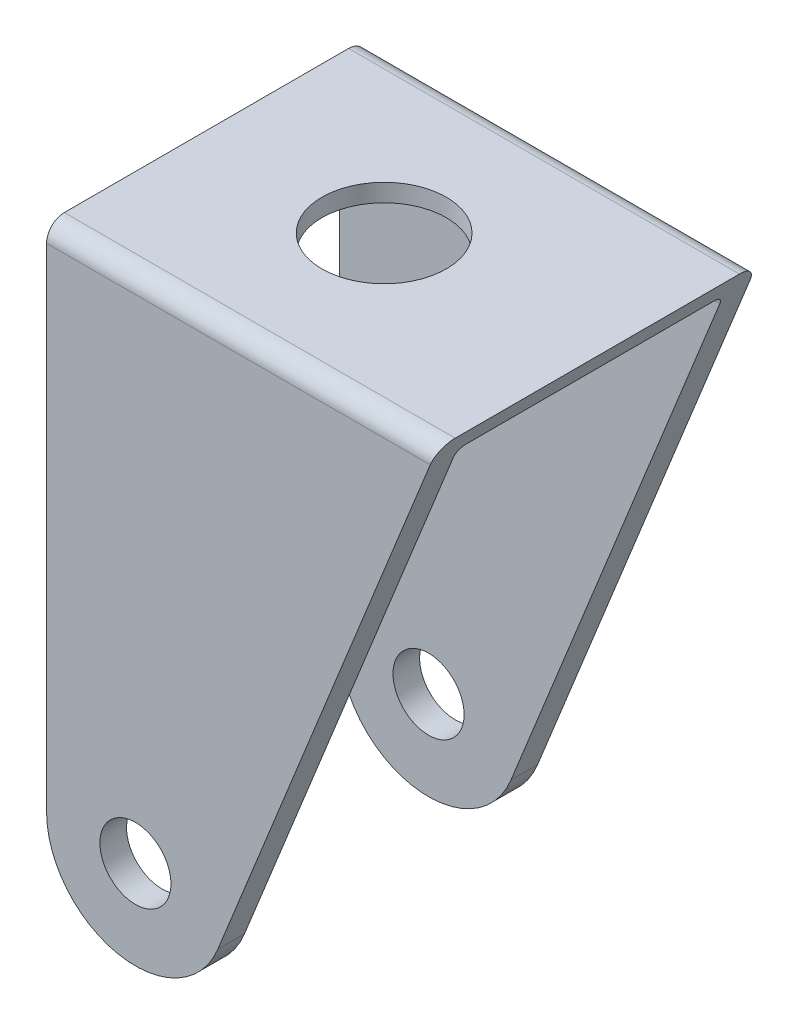
from build123d import *

# Parameters (mm, degrees)
SKETCH1_R           = 4
BOSS_EXTRUDE1_DEPTH = 36
CUT_EXTRUDE1_DEPTH  = 57
FILLET1_R           = 2
SKETCH3_R           = 7
CUT_EXTRUDE2_DEPTH  = 57


with BuildPart() as part:
    # Sketch1 → Boss-Extrude1 (new body)
    with BuildSketch(Plane.XY):
        with BuildLine():
            Line((0, 0), (0, -57.458281391))
            ThreePointArc((0, -57.458281391), (8.091910046, -67.274553225), (19.271838546, -61.204347325))
            Line((19.271838546, -61.204347325), (44, 0))
            Line((44, 0), (0, 0))
        make_face()
        with Locations((10, -57.458281391)):
            Circle(SKETCH1_R, mode=Mode.SUBTRACT)
    extrude(amount=-BOSS_EXTRUDE1_DEPTH)

    # Sketch2 → Cut-Extrude1 (cut)
    with BuildSketch(Plane.ZY):
        with BuildLine():
            Line((-32, -2), (-4, -2))
            ThreePointArc((-4, -2), (-3.292893219, -2.292893219), (-3, -3))
            Line((-3, -3), (-3, -57.458281391))
            Line((-3, -57.458281391), (-3, -71.28436633))
            Line((-3, -71.28436633), (-33, -71.28436633))
            Line((-33, -71.28436633), (-33, -57.458281391))
            Line((-33, -57.458281391), (-33, -3))
            ThreePointArc((-33, -3), (-32.707106781, -2.292893219), (-32, -2))
        make_face()
    extrude(amount=-CUT_EXTRUDE1_DEPTH, mode=Mode.SUBTRACT)

    # Fillet1
    fillet1_edges = [part.edges().sort_by_distance(p)[0] for p in [
        (22, 0, -36),
        (22, 0, 0),
    ]]
    fillet(fillet1_edges, radius=FILLET1_R)

    # Sketch3 → Cut-Extrude2 (cut)
    with BuildSketch(Plane(origin=(0, 0, 0), x_dir=(1, 0, 0), z_dir=(0, 1, 0))):
        with Locations(Location((20, 18, 0), (0, 0, 270))):
            Circle(SKETCH3_R)
    extrude(amount=-CUT_EXTRUDE2_DEPTH, mode=Mode.SUBTRACT)


solid = part.part
